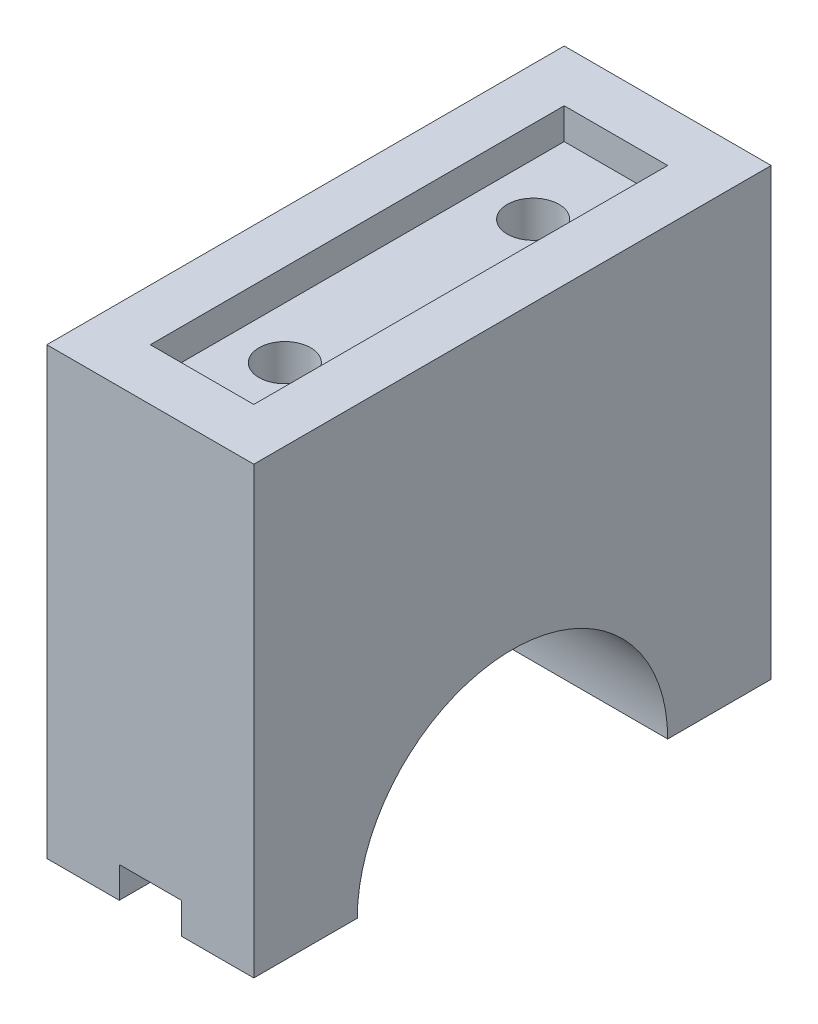
from build123d import *

# Parameters (mm, degrees)
SKETCH1_W                  = 20
SKETCH1_H                  = 43
BOSS_EXTRUDE1_DEPTH        = 50
SKETCH2_R                  = 15
CUT_EXTRUDE1_DEPTH         = 50
CUT_EXTRUDE2_DEPTH         = 5
SKETCH4_W                  = 6
SKETCH4_H                  = 5
CUT_EXTRUDE3_DEPTH         = 3
SIZE_MM_DOWEL_HOLE_1_D     = 4.2
SIZE_MM_DOWEL_HOLE_1_DEPTH = 14.2
SIZE_MM_DOWEL_HOLE_1_TIP   = 1.2618073
SKETCH8_W                  = 10
SKETCH8_H                  = 40
CUT_EXTRUDE4_DEPTH         = 3
SIZE_MM_DOWEL_HOLE_2_D     = 5
SIZE_MM_DOWEL_HOLE_2_DEPTH = 17.1
SIZE_MM_DOWEL_HOLE_2_TIP   = 1.502151548


with BuildPart() as part:
    # Sketch1 → Boss-Extrude1 (new body)
    with BuildSketch(Plane.XY):
        Rectangle(SKETCH1_W, SKETCH1_H)
    extrude(amount=BOSS_EXTRUDE1_DEPTH)

    # Sketch2 → Cut-Extrude1 (cut)
    with BuildSketch(Plane(origin=(10, 0, 0), x_dir=(0, 0, -1), z_dir=(1, 0, 0))):
        with Locations((-25, -21.5)):
            Circle(SKETCH2_R)
    extrude(amount=-CUT_EXTRUDE1_DEPTH, mode=Mode.SUBTRACT)

    # Sketch3 → Cut-Extrude2 (cut)
    with BuildSketch(Plane.ZY.offset(10)):
        with BuildLine():
            Line((19.083920217, -4.5), (30.916079783, -4.5))
            ThreePointArc((30.916079783, -4.5), (25, -39.5), (19.083920217, -4.5))
        make_face()
    extrude(amount=-CUT_EXTRUDE2_DEPTH, mode=Mode.SUBTRACT)

    # Sketch4 → Cut-Extrude3 (cut)
    with BuildSketch(Plane.XZ.offset(21.5)):
        with Locations((0, 2.5)):
            Rectangle(SKETCH4_W, SKETCH4_H)
        with Locations((0, 47.5)):
            Rectangle(SKETCH4_W, SKETCH4_H)
    extrude(amount=-CUT_EXTRUDE3_DEPTH, mode=Mode.SUBTRACT)

    # Size mm Dowel hole 1
    with Locations(Plane(origin=(0, -21.5, 0), x_dir=(-1, 0, 0), z_dir=(0, -1, 0))):
        with Locations((6, -4), (-6, -4), (6, -46), (-6, -46)):
            Hole(SIZE_MM_DOWEL_HOLE_1_D / 2, depth=SIZE_MM_DOWEL_HOLE_1_DEPTH)
            with Locations((0, 0, -(SIZE_MM_DOWEL_HOLE_1_DEPTH + SIZE_MM_DOWEL_HOLE_1_TIP / 2))):  # 118° drill point
                Cone(0, SIZE_MM_DOWEL_HOLE_1_D / 2, SIZE_MM_DOWEL_HOLE_1_TIP, mode=Mode.SUBTRACT)

    # Sketch8 → Cut-Extrude4 (cut)
    with BuildSketch(Plane(origin=(0, 21.5, 0), x_dir=(1, 0, 0), z_dir=(0, 1, 0))):
        with Locations((0, -25)):
            Rectangle(SKETCH8_W, SKETCH8_H)
    extrude(amount=-CUT_EXTRUDE4_DEPTH, mode=Mode.SUBTRACT)

    # Size mm Dowel hole 2
    with Locations(Plane(origin=(0, 18.5, 0), x_dir=(1, 0, 0), z_dir=(0, 1, 0))):
        with Locations((0, -13), (0, -37)):
            Hole(SIZE_MM_DOWEL_HOLE_2_D / 2, depth=SIZE_MM_DOWEL_HOLE_2_DEPTH)
            with Locations((0, 0, -(SIZE_MM_DOWEL_HOLE_2_DEPTH + SIZE_MM_DOWEL_HOLE_2_TIP / 2))):  # 118° drill point
                Cone(0, SIZE_MM_DOWEL_HOLE_2_D / 2, SIZE_MM_DOWEL_HOLE_2_TIP, mode=Mode.SUBTRACT)


solid = part.part
